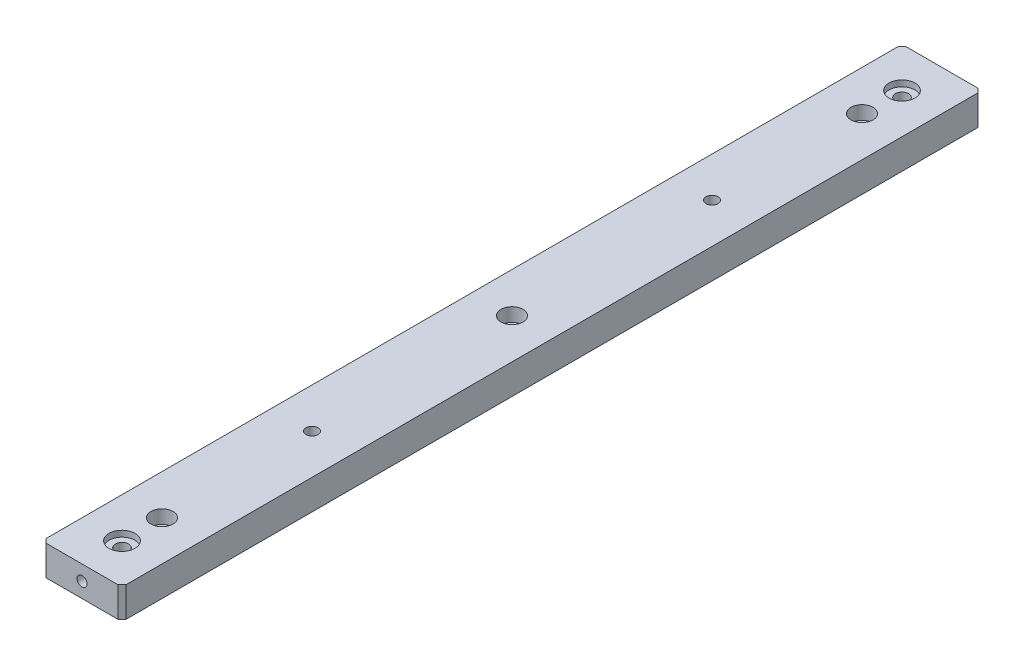
SolidWorks part; units mm, degrees
material "A5052"
ref_plane "Front Plane" through (0, 0, 0) normal (0, 0, 1) x (1, 0, 0)
ref_plane "Top Plane" through (0, 0, 0) normal (0, 1, 0) x (1, 0, 0)
ref_plane "Right Plane" through (0, 0, 0) normal (1, 0, 0) x (0, 0, -1)
sketch "Sketch1" plane through (0, 0, 0) normal (0, 1, 0) x (1, 0, 0)
  line L1 (20, 215) -> (-20, 215)
  line L2 (20, 215) -> (20, -215)
  line L3 (20, -215) -> (-20, -215)
  line L4 (-20, 215) -> (-20, -215)
  line L5 (20, 215) -> (-20, -215) construction
  line L6 (20, -215) -> (-20, 215) construction
  point P0 (0, 0)
  dimension "D1" = 40
  dimension "D2" = 430
extrude "Boss-Extrude1" add sketch "Sketch1" along normal mid plane 15
sketch "Sketch2" plane through (0, 7.5, 0) normal (0, 1, 0) x (1, 0, 0)
  line L0 (0, 0) -> (0, 195) construction
  line L1 (20, 215) -> (-20, 215) construction
  line L2 (0, 0) -> (43.891, 0) construction
  circle A0 centre (0, 195) radius 6.5
  circle A1 centre (0, -195) radius 6.5
  dimension "D1" = 13
  dimension "D2" = 20
extrude "Cut-Extrude1" cut sketch "Sketch2" against normal blind 3
hole_wizard "Hex socket cap screw hole type 1" positions "Sketch3" profile "Sketch4" counterbore size "M6" standard "GB" end condition through all
sketch "Sketch3" plane through (0, -7.5, 0) normal (0, -1, 0) x (-1, 0, 0)
  point P0 (0, -195)
  point P3 (0, 195)
sketch "Sketch4" plane through (0, -7.5, 195) normal (1, 0, 0) x (0, 0, -1)
  line L0 (0, 0) -> (0, 15)
  line L1 (0, 15) -> (3.3, 15)
  line L3 (3.3, 15) -> (3.3, 6.8)
  line L4 (3.3, 6.8) -> (5.5, 6.8)
  line L5 (5.5, 6.8) -> (5.5, 0)
  line L7 (5.5, 0) -> (0, 0)
  line L11 (0, -6.35) -> (0, 107.95) construction
  dimension "通孔孔直径" = 6.6
  dimension "通孔孔深度" = 15
  dimension "柱形沉头孔直径" = 11
  dimension "柱形沉头孔深度" = 6.8
hole_wizard "M5 Tapped Hole1" positions "Sketch5" profile "Sketch6" tap size "M5" standard "GB"
sketch "Sketch5" plane through (-20, 0, 0) normal (-1, 0, 0) x (0, 0, 1)
  line L1 (0, 0) -> (-195, 0) construction
  line L4 (0, 0) -> (0, 27.881) construction
  point P0 (-195, 0)
  point P21 (195, 0)
  point P23 (-65, 0)
  point P25 (65, 0)
  dimension "D1" = 130
  dimension "D2" = 130
sketch "Sketch6" plane through (-20, 0, -195) normal (0, 1, 0) x (0, 0, 1)
  line L0 (0, 0) -> (0, 16.2618)
  line L1 (0, 16.2618) -> (2.1, 15)
  line L2 (2.1, 15) -> (2.1, 0)
  line L5 (2.1, 0) -> (0, 0)
  line L10 (0, 16.2618) -> (-2.1, 15) construction
  line L11 (0, -6.35) -> (0, 107.95) construction
  dimension "螺纹孔钻头直径" = 4.2
  dimension "螺纹孔钻头深度" = 15
  dimension "导头角度" = 118
cosmetic thread "Hole thread 1" parameters "D1"=10, "D2"=5
cosmetic thread "Hole thread 2" parameters "D1"=10, "D2"=5
cosmetic thread "Hole thread 3" parameters "D1"=10, "D2"=5
cosmetic thread "Hole thread 6" parameters "D1"=10, "D2"=5
chamfer "Chamfer1" distance 2 angle 45 4 edges at (20, 0, -215) (-20, 0, -215) (20, 0, 215) (-20, 0, 215)
hole_wizard "Hex socket cap screw hole type 2" positions "Sketch7" profile "Sketch8" counterbore size "M6" standard "GB" end condition through all
sketch "Sketch7" plane through (0, 7.5, 0) normal (0, 1, 0) x (1, 0, 0)
  line L0 (0, 0) -> (20, 0) construction
  line L1 (20, -213) -> (20, 213) construction
  line L4 (0, 0) -> (0, 175) construction
  point P0 (0, 175)
  point P20 (0, -175)
  point P23 (0, 0)
  dimension "D1" = 350
sketch "Sketch8" plane through (0, 7.5, -175) normal (1, 0, 0) x (0, 0, 1)
  line L0 (0, 0) -> (0, 15)
  line L1 (0, 15) -> (3.3, 15)
  line L3 (3.3, 15) -> (3.3, 6.8)
  line L4 (3.3, 6.8) -> (5.5, 6.8)
  line L5 (5.5, 6.8) -> (5.5, 0)
  line L7 (5.5, 0) -> (0, 0)
  line L11 (0, -6.35) -> (0, 107.95) construction
  dimension "通孔孔直径" = 6.6
  dimension "通孔孔深度" = 15
  dimension "柱形沉头孔直径" = 11
  dimension "柱形沉头孔深度" = 6.8
hole_wizard "M6 Tapped Hole1" positions "Sketch9" profile "Sketch10" tap size "M6" standard "GB"
sketch "Sketch9" plane through (0, 0, 215) normal (0, 0, 1) x (1, 0, 0)
  point P0 (0, 0)
sketch "Sketch10" plane through (0, 0, 215) normal (1, 0, 0) x (0, -1, 0)
  line L0 (0, 0) -> (0, 14.5022)
  line L1 (0, 14.5022) -> (2.5, 13)
  line L2 (2.5, 13) -> (2.5, 0)
  line L5 (2.5, 0) -> (0, 0)
  line L10 (0, 14.5022) -> (-2.5, 13) construction
  line L11 (0, -6.35) -> (0, 107.95) construction
  dimension "螺纹孔钻头直径" = 5
  dimension "螺纹孔钻头深度" = 13
  dimension "导头角度" = 118
cosmetic thread "Hole thread 4" parameters "D1"=10, "D2"=6
hole_wizard "M6 Tapped Hole2" positions "Sketch11" profile "Sketch12" tap size "M6" standard "GB"
sketch "Sketch11" plane through (0, 0, -215) normal (0, 0, -1) x (-1, 0, 0)
  point P0 (0, 0)
sketch "Sketch12" plane through (0, 0, -215) normal (1, 0, 0) x (0, 1, 0)
  line L0 (0, 0) -> (0, 14.5022)
  line L1 (0, 14.5022) -> (2.5, 13)
  line L2 (2.5, 13) -> (2.5, 0)
  line L5 (2.5, 0) -> (0, 0)
  line L10 (0, 14.5022) -> (-2.5, 13) construction
  line L11 (0, -6.35) -> (0, 107.95) construction
  dimension "螺纹孔钻头直径" = 5
  dimension "螺纹孔钻头深度" = 13
  dimension "导头角度" = 118
cosmetic thread "Hole thread 5" parameters "D1"=10, "D2"=6
hole_wizard "Ø6.0 (6) Diameter Hole1" positions "Sketch13" profile "Sketch14" hole size "Ø6.0" standard "GB"
sketch "Sketch13" plane through (0, -7.5, 0) normal (0, -1, 0) x (-1, 0, 0)
  line L0 (0, 0) -> (17.764, 0) construction
  point P0 (0, 100)
  point P2 (0, -100)
  dimension "D1" = 200
sketch "Sketch14" plane through (0, -7.5, -100) normal (1, 0, 0) x (0, 0, -1)
  line L0 (0, 0) -> (0, 18.8026)
  line L1 (0, 18.8026) -> (3, 17)
  line L2 (3, 17) -> (3, 0)
  line L5 (3, 0) -> (0, 0)
  line L10 (0, 18.8026) -> (-3, 17) construction
  line L11 (0, -6.35) -> (0, 107.95) construction
  dimension "孔直径" = 6
  dimension "孔深度" = 17
  dimension "导头角度" = 118
sketch "Sketch15" plane through (0, -7.5, 0) normal (0, -1, 0) x (1, 0, 0)
  line L0 (20, 213) -> (20, -213) construction
  line L1 (20, 85) -> (10, 85)
  line L2 (20, 85) -> (20, 135)
  line L3 (20, 135) -> (10, 135)
  line L4 (10, 85) -> (10, 135)
  line L5 (-18, 215) -> (18, 215) construction
  dimension "D1" = 10
  dimension "D2" = 80
  dimension "D3" = 50
extrude "Cut-Extrude2" [suppressed] cut sketch "Sketch15" against normal through all
fillet "Fillet1" [suppressed] radius 3
chamfer "Chamfer2" [suppressed] distance 3 angle 45
